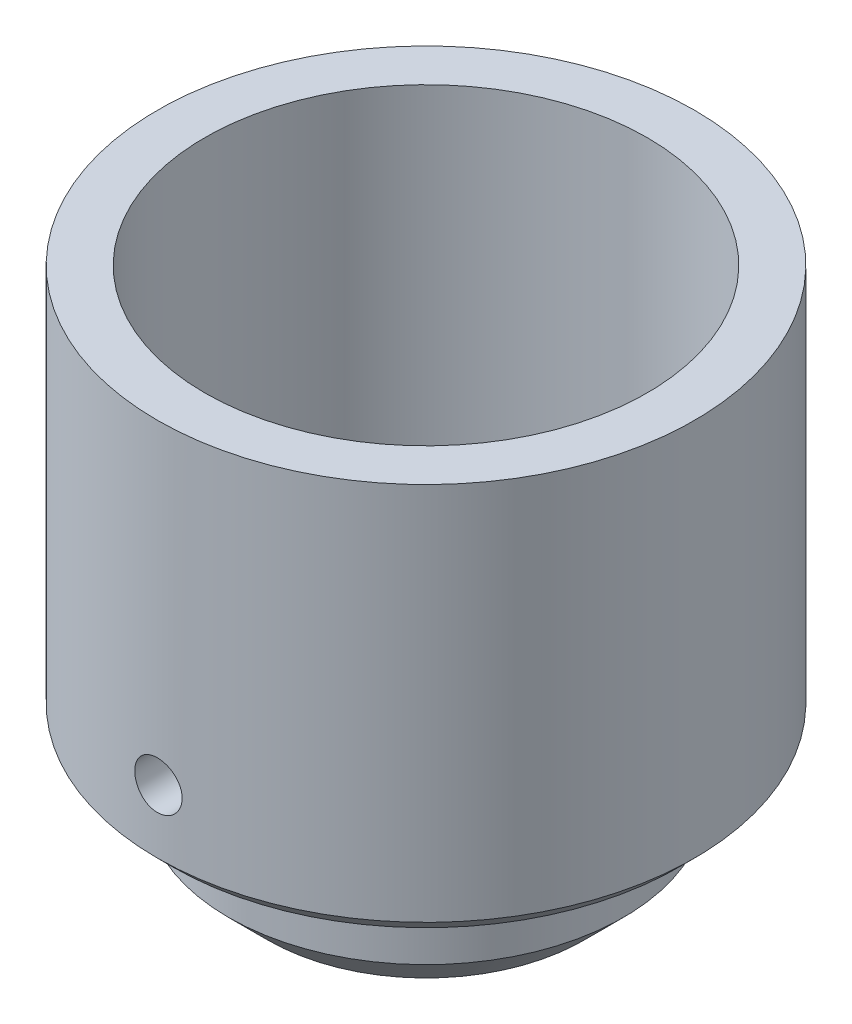
from build123d import *

# Parameters (mm, degrees)
M6_TAPPED_HOLE1_D     = 5
M6_TAPPED_HOLE1_DEPTH = 5
M6_TAPPED_HOLE1_TIP   = 1.502151548
SKETCH4_R             = 1.5
CUT_EXTRUDE1_DEPTH    = 35


with BuildPart() as part:
    # Sketch1 → Revolve1 (revolve)
    with BuildSketch(Plane.XY, mode=Mode.PRIVATE) as revolve1_sk:
        Polygon((0, 0), (-10, 0), (-12.5, 2.5), (-12.5, 7), (-16, 7), (-17, 8), (-17, 32), (-14, 32), (-14, 10), (0, 10), align=None)
    revolve(revolve1_sk.sketch.rotate(Axis((0, 19.380505724, 0), (0, -1, 0)), 270), axis=Axis((0, 19.380505724, 0), (0, -1, 0)))

    # M6 Tapped Hole1
    with Locations(Plane(origin=(0, 10, 0), x_dir=(1, 0, 0), z_dir=(0, 1, 0))):
        with Locations((0, 0)):
            Hole(M6_TAPPED_HOLE1_D / 2, depth=M6_TAPPED_HOLE1_DEPTH)
            with Locations((0, 0, -(M6_TAPPED_HOLE1_DEPTH + M6_TAPPED_HOLE1_TIP / 2))):  # 118° drill point
                Cone(0, M6_TAPPED_HOLE1_D / 2, M6_TAPPED_HOLE1_TIP, mode=Mode.SUBTRACT)

    # Sketch4 → Cut-Extrude1 (cut, symmetric)
    with BuildSketch(Plane.XY):
        with Locations((0, 12)):
            Circle(SKETCH4_R)
    extrude(amount=CUT_EXTRUDE1_DEPTH, both=True, mode=Mode.SUBTRACT)


solid = part.part
